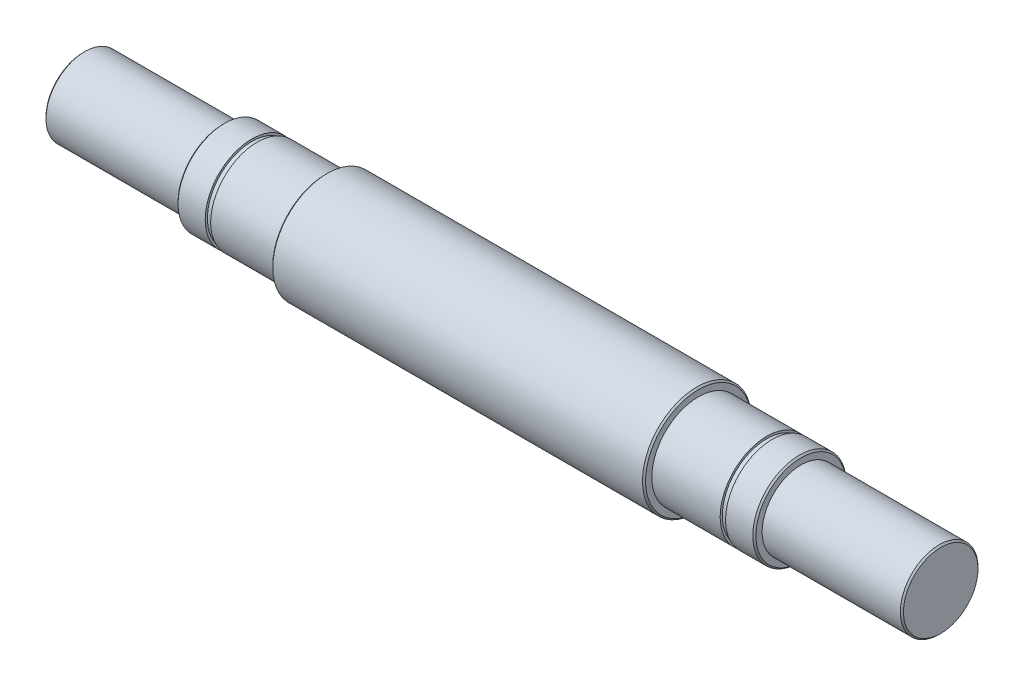
from build123d import *

# Parameters (mm, degrees)
CHAMFER_1_SIZE      = 0.5
CUT_EXTRUDE_START   = -11
CUT_EXTRUDE_1_DEPTH = 10
SKETCH_11_R         = 20.368798622
SKETCH_11_R_2       = 14.3
CUT_EXTRUDE_3_DEPTH = 1.75
CHAMFER_3_SIZE      = 0.5


with BuildPart() as part:
    # 草图1 → 旋转1 (revolve)
    with BuildSketch(Plane(origin=(0, 0, 0), x_dir=(-1, 0, 0), z_dir=(0, 0, -1)), mode=Mode.PRIVATE) as revolve_1_sk:
        Polygon((-60, 17.5), (60, 17.5), (60, 15), (93, 15), (93, 12.5), (138, 12.5), (138, 0), (-138, 0), (-138, 12.5), (-93, 12.5), (-93, 15), (-60, 15), align=None)
    revolve(revolve_1_sk.sketch.rotate(Axis((70, 0, 0), (-1, 0, 0)), 270), axis=Axis((70, 0, 0), (-1, 0, 0)))

    # 倒角1
    chamfer_1_edges = [part.edges().sort_by_distance(p)[0] for p in [
        (-138, 0, -12.5),
        (-93, 0, -15),
        (-60, 0, -17.5),
        (60, 0, -17.5),
        (93, 0, -15),
    ]]
    chamfer(chamfer_1_edges, length=CHAMFER_1_SIZE)

    # 草图2 → 切除-拉伸1 (cut)
    with BuildSketch(Plane.XY.offset(CUT_EXTRUDE_START)):
        with BuildLine():
            Line((-77, 4), (-65, 4))
            ThreePointArc((-65, 4), (-61, 0), (-65, -4))
            Line((-65, -4), (-77, -4))
            ThreePointArc((-77, -4), (-81, 0), (-77, 4))
        make_face()
        with BuildLine():
            Line((65, 4), (77, 4))
            ThreePointArc((77, 4), (81, 0), (77, -4))
            Line((77, -4), (65, -4))
            ThreePointArc((65, -4), (61, 0), (65, 4))
        make_face()
    extrude(amount=-CUT_EXTRUDE_1_DEPTH, mode=Mode.SUBTRACT)

    # 草图11 → 切除-拉伸3 (cut)
    with BuildSketch(Plane(origin=(82, 0, 0), x_dir=(0, 0, -1), z_dir=(1, 0, 0))):
        Circle(SKETCH_11_R)
        Circle(SKETCH_11_R_2, mode=Mode.SUBTRACT)
    cut_extrude_3 = extrude(amount=CUT_EXTRUDE_3_DEPTH, mode=Mode.SUBTRACT)

    # 镜向1: 切除-拉伸3 across plane
    add(cut_extrude_3.mirror(Plane(origin=(0, 0, 0), x_dir=(0, 0, 1), z_dir=(1, 0, 0))), mode=Mode.SUBTRACT)

    # 倒角3
    chamfer_3_edges = [part.edges().sort_by_distance(p)[0] for p in [
        (138, 0, -12.5),
    ]]
    chamfer(chamfer_3_edges, length=CHAMFER_3_SIZE)


solid = part.part
